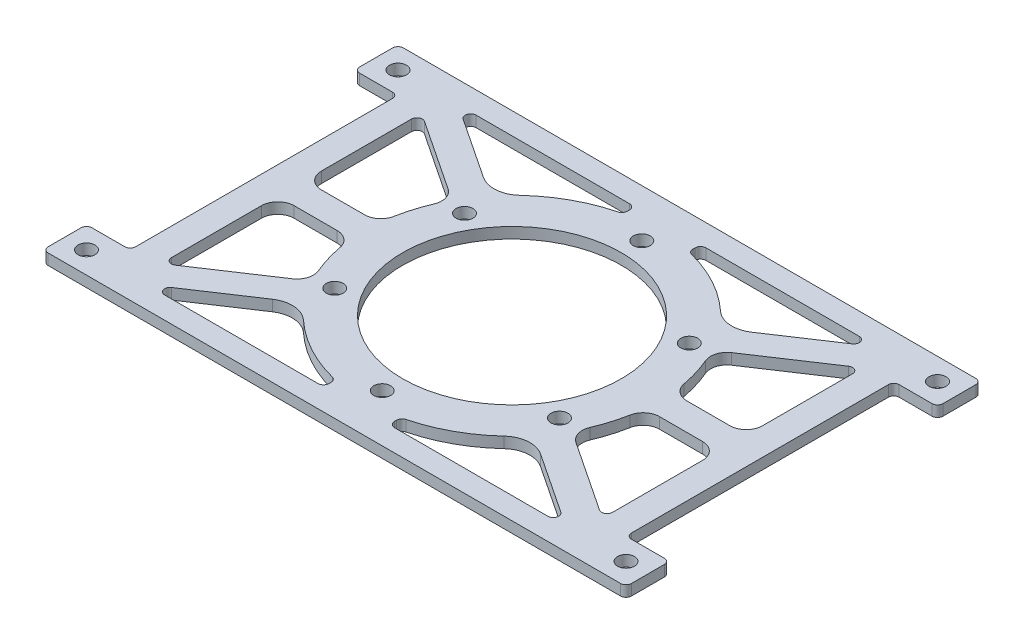
SolidWorks part; units mm, degrees
material "Thornel Mat VMA"
ref_plane "前视基准面" through (0, 0, 0) normal (0, 0, 1) x (1, 0, 0)
ref_plane "上视基准面" through (0, 0, 0) normal (0, 1, 0) x (1, 0, 0)
ref_plane "右视基准面" through (0, 0, 0) normal (1, 0, 0) x (0, 0, -1)
other "Configuration Table"
sketch "草图1" plane through (0, 0, 0) normal (0, 1, 0) x (1, 0, 0)
  line L0 (0, 0) -> (99.9087, 0) construction
  line L1 (0, 0) -> (0, 82.5816) construction
  line L2 (0, 0) -> (49.3634, 28.5) construction
  line L3 (20.5681, 11.875) -> (0, 0) construction
  line L4 (-53.3634, 32.5) -> (53.3634, 32.5)
  line L5 (53.3634, 32.5) -> (53.3634, 24.5)
  line L6 (53.3634, 24.5) -> (45.3634, 24.5)
  line L7 (45.3634, 24.5) -> (45.3634, -24.5)
  line L8 (53.3634, -24.5) -> (45.3634, -24.5)
  line L9 (53.3634, -32.5) -> (53.3634, -24.5)
  line L10 (-53.3634, -32.5) -> (53.3634, -32.5)
  line L11 (-53.3634, -32.5) -> (-53.3634, -24.5)
  line L12 (-53.3634, -24.5) -> (-45.3634, -24.5)
  line L13 (-45.3634, 24.5) -> (-45.3634, -24.5)
  line L14 (-53.3634, 24.5) -> (-45.3634, 24.5)
  line L15 (-53.3634, 32.5) -> (-53.3634, 24.5)
  line L17 (-38.3634, 28.5) -> (-6, 28.5)
  line L18 (-38.3634, 28.5) -> (-21.0059, 16.9633)
  line L19 (-23.7735, 12.7992) -> (-40.3634, 23.8256)
  line L20 (-40.3634, 23.8256) -> (-40.3634, 2.5)
  line L21 (-40.3634, 2.5) -> (-26.884, 2.5)
  line L22 (-38.3634, -28.5) -> (-6, -28.5)
  line L23 (-38.3634, -28.5) -> (-21.0059, -16.9633)
  line L24 (-23.7735, -12.7992) -> (-40.3634, -23.8256)
  line L25 (-40.3634, -2.5) -> (-26.884, -2.5)
  line L26 (-40.3634, -23.8256) -> (-40.3634, -2.5)
  line L27 (38.3634, -28.5) -> (21.0059, -16.9633)
  line L28 (23.7735, -12.7992) -> (40.3634, -23.8256)
  line L29 (40.3634, -23.8256) -> (40.3634, -2.5)
  line L30 (40.3634, -2.5) -> (26.884, -2.5)
  line L31 (40.3634, 2.5) -> (26.884, 2.5)
  line L32 (38.3634, 28.5) -> (21.0059, 16.9633)
  line L33 (23.7735, 12.7992) -> (40.3634, 23.8256)
  line L34 (40.3634, 23.8256) -> (40.3634, 2.5)
  line L35 (-6, 28.5) -> (-6, 26.3249)
  line L36 (6, 28.5) -> (6, 26.3249)
  line L37 (6, -28.5) -> (6, -26.3249)
  line L38 (-6, -28.5) -> (-6, -26.3249)
  line L39 (-36.3312, 24.1474) -> (-24.0123, 15.9597) construction
  line L40 (6, 28.5) -> (38.3634, 28.5)
  line L41 (6, -28.5) -> (38.3634, -28.5)
  circle A0 centre (0, 0) radius 57 construction
  circle A1 centre (49.3634, 28.5) radius 1.55
  circle A2 centre (49.3634, -28.5) radius 1.55
  circle A3 centre (-49.3634, 28.5) radius 1.55
  circle A4 centre (-49.3634, -28.5) radius 1.55
  circle A5 centre (0, 0) radius 23.75 construction
  circle A6 centre (20.5681, 11.875) radius 1.55
  circle A10 centre (0, 0) radius 20
  circle A11 centre (20.5681, -11.875) radius 1.55
  circle A16 centre (0, -23.75) radius 1.55
  circle A21 centre (-20.5681, -11.875) radius 1.55
  circle A26 centre (-20.5681, 11.875) radius 1.55
  arc A31 (-23.7735, 12.7992) -> (-26.884, 2.5) centre (0, 0) ccw
  arc A32 (-6, 26.3249) -> (-21.0059, 16.9633) centre (0, 0) ccw
  arc A33 (-26.884, -2.5) -> (-23.7735, -12.7992) centre (0, 0) ccw
  arc A34 (-21.0059, -16.9633) -> (-6, -26.3249) centre (0, 0) ccw
  arc A35 (6, -26.3249) -> (21.0059, -16.9633) centre (0, 0) ccw
  arc A36 (23.7735, -12.7992) -> (26.884, -2.5) centre (0, 0) ccw
  arc A37 (26.884, 2.5) -> (23.7735, 12.7992) centre (0, 0) ccw
  arc A38 (21.0059, 16.9633) -> (6, 26.3249) centre (0, 0) ccw
  circle A39 centre (0, 23.75) radius 1.55
  point P16 (-21.0059, 13.141)
  point P19 (0, 0)
  point P25 (0, 0)
  point P30 (45.3634, 0)
  point P34 (0, -32.5)
  point P39 (0, 32.5)
  point P46 (0, 0)
  point P72 (0, 0)
  dimension "D1" = 114
  dimension "D3" = 3.1
  dimension "D4" = 47.5
  dimension "D6" = 40
  dimension "D7" = 4
  dimension "D11" = 6
  dimension "D13" = 4
  dimension "D19" = 54
  dimension "D2" = 30
  dimension "D5" = 30
  dimension "D8" = 4
  dimension "D9" = 4
  dimension "D10" = 4
  dimension "D15" = 15
  dimension "D16" = 5
  dimension "D17" = 2.5
  dimension "D18" = 5
  dimension "D20" = 6
extrude "凸台-拉伸1" add sketch "草图1" along normal blind 2
fillet "圆角1" radius 1 28 edges at (-6, 1, -28.5) (-6, 1, -26.3249) (6, 1, -26.3249) (6, 1, -28.5) (6, 1, 28.5) (6, 1, 26.3249) (-6, 1, 28.5) (-6, 1, 26.3249) (40.3634, 1, 23.8256) (40.3634, 1, -23.8256) (-40.3634, 1, -23.8256) (-40.3634, 1, 23.8256) (-38.3634, 1, 28.5) (38.3634, 1, 28.5) (38.3634, 1, -28.5) (-38.3634, 1, -28.5) (53.3634, 1, -32.5) (53.3634, 1, -24.5) (45.3634, 1, -24.5) (45.3634, 1, 24.5) (53.3634, 1, 24.5) (53.3634, 1, 32.5) (-53.3634, 1, 32.5) (-53.3634, 1, 24.5) (-45.3634, 1, 24.5) (-45.3634, 1, -24.5) (-53.3634, 1, -32.5) (-53.3634, 1, -24.5)
fillet "圆角2" radius 3 12 edges at (-23.7735, 1, -12.7992) (-40.3634, 1, -2.5) (-26.884, 1, -2.5) (-26.884, 1, 2.5) (-40.3634, 1, 2.5) (-23.7735, 1, 12.7992) (23.7735, 1, 12.7992) (26.884, 1, 2.5) (26.884, 1, -2.5) (23.7735, 1, -12.7992) (40.3634, 1, -2.5) (40.3634, 1, 2.5)
fillet "圆角3" radius 5 4 edges at (21.0059, 1, -16.9633) (21.0059, 1, 16.9633) (-21.0059, 1, 16.9633) (-21.0059, 1, -16.9633)
